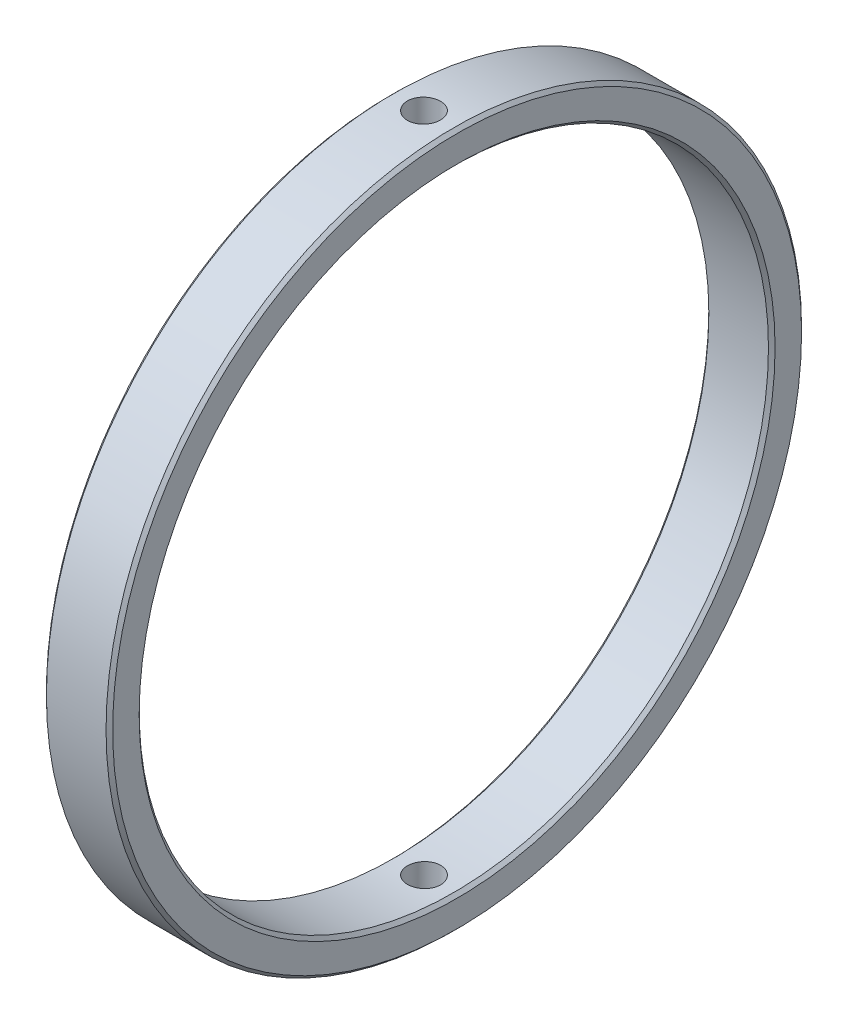
SolidWorks part; units mm, degrees
material "45"
ref_plane "前视基准面" through (0, 0, 0) normal (0, 0, 1) x (1, 0, 0)
ref_plane "上视基准面" through (0, 0, 0) normal (0, 1, 0) x (1, 0, 0)
ref_plane "右视基准面" through (0, 0, 0) normal (1, 0, 0) x (0, 0, -1)
sketch "草图1" plane through (0, 0, 0) normal (1, 0, 0) x (0, 0, -1)
  circle A0 centre (0, 0) radius 47.5
  circle A1 centre (0, 0) radius 52.5
  dimension "D1" = 95
  dimension "D2" = 105
extrude "凸台-拉伸1" add sketch "草图1" along normal mid plane 10
chamfer "倒角1" distance 0.5 angle 45 4 edges at (-5, 0, -52.5) (5, 0, -52.5) (-5, 0, -47.5) (5, 0, -47.5)
ref_plane "基准面1" through (0, 52.5, 0) normal (0, 1, 0) x (1, 0, 0)
hole_wizard "M6 螺纹孔1" positions "草图2" profile "草图3" tap size "M6" standard "GB" end condition through all
sketch "草图2" plane through (0, 52.5, 0) normal (0, 1, 0) x (1, 0, 0)
  point P0 (0, 0)
sketch "草图3" plane through (0, 52.5, 0) normal (1, 0, 0) x (0, 0, 1)
  line L0 (0, 0) -> (0, 105)
  line L1 (0, 105) -> (2.5, 105)
  line L2 (2.5, 105) -> (2.5, 0)
  line L5 (2.5, 0) -> (0, 0)
  line L11 (0, -6.35) -> (0, 107.95) construction
  dimension "通孔螺纹孔钻头直径" = 5
  dimension "通孔螺纹孔钻头深度" = 105
cosmetic thread "孔螺蚊线1" parameters "D2"=6
equation "\"XMMCDM\"= \"QC名称代码\""
